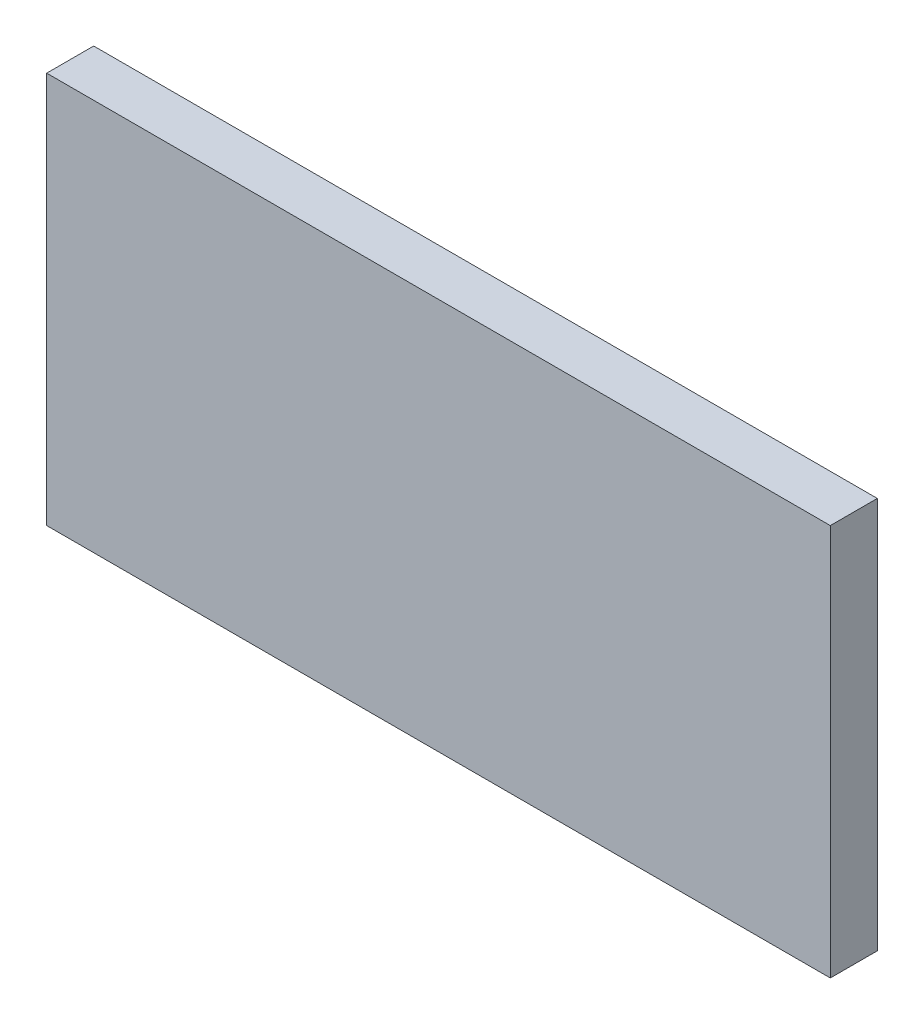
from build123d import *

# Parameters (mm, degrees)
SKETCH_1_W      = 200
SKETCH_1_H      = 100
EXTRUDE_1_DEPTH = 12


with BuildPart() as part:
    # 草图1 → 凸台-拉伸1 (new body)
    with BuildSketch(Plane.XY):
        Rectangle(SKETCH_1_W, SKETCH_1_H)
    extrude(amount=EXTRUDE_1_DEPTH)


solid = part.part
